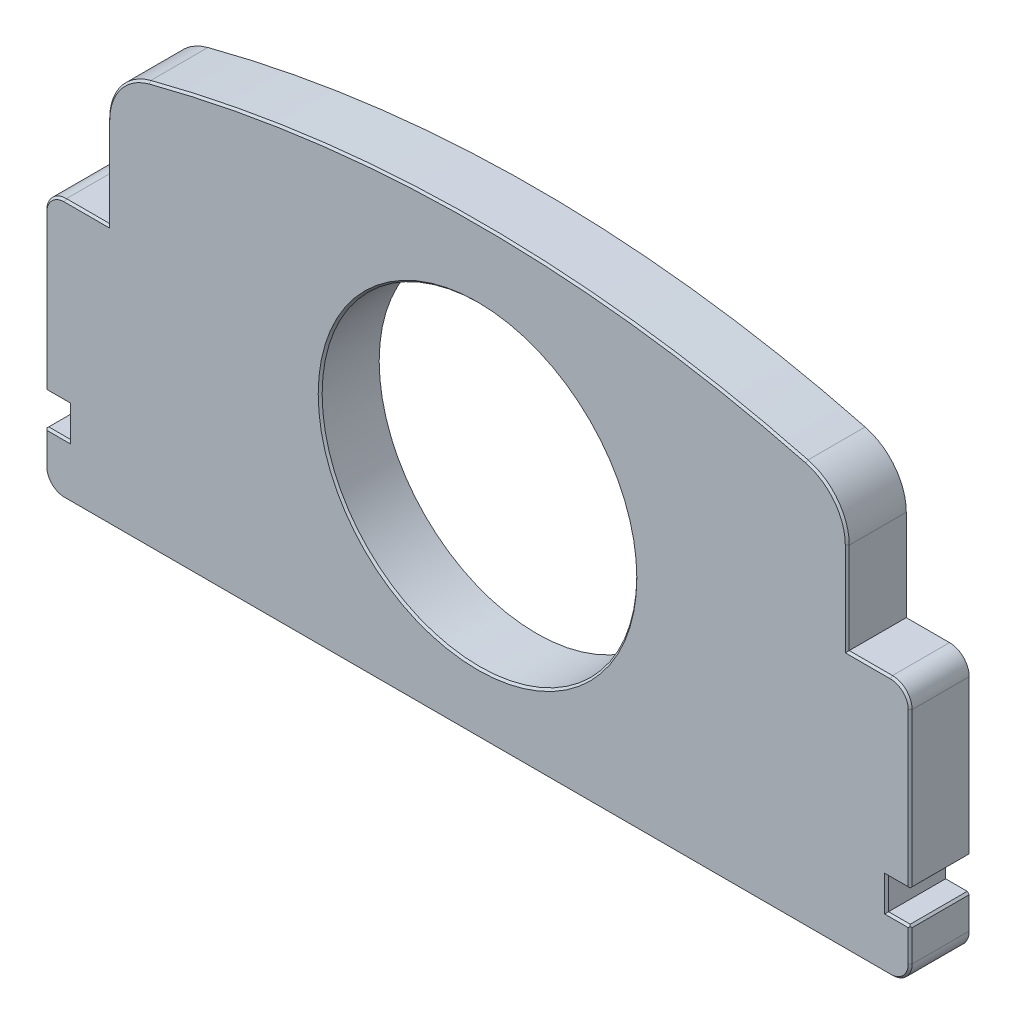
SolidWorks part; units mm, degrees
material "6061 合金"
ref_plane "前视基准面" through (0, 0, 0) normal (0, 0, 1) x (1, 0, 0)
ref_plane "上视基准面" through (0, 0, 0) normal (0, 1, 0) x (1, 0, 0)
ref_plane "右视基准面" through (0, 0, 0) normal (1, 0, 0) x (0, 0, -1)
sketch "草图1" plane through (0, 0, 0) normal (0, 0, 1) x (1, 0, 0)
  line L1 (-110, 121) -> (110, 121)
  line L2 (-110, 121) -> (-110, 0)
  line L3 (-110, 0) -> (110, 0)
  line L4 (110, 121) -> (110, 0)
  dimension "D1" = 220
  dimension "D2" = 121
extrude "凸台-拉伸1" add sketch "草图1" along normal mid plane 15
sketch "草图4" plane through (0, 0, 7.5) normal (0, 0, 1) x (1, 0, 0)
  line L0 (-94, 66) -> (-110, 66)
  line L1 (-110, 121) -> (-110, 0) construction
  line L2 (-110, 122.2) -> (110, 122.2)
  line L3 (110, 122.2) -> (110, 66)
  line L4 (110, 0) -> (110, 121) construction
  line L5 (-94, 66) -> (-94, 89.2057)
  line L6 (94, 66) -> (94, 89.2057)
  line L10 (0, 0) -> (0, 121) construction
  line L12 (110, 66) -> (94, 66)
  line L13 (-110, 66) -> (-110, 122.2)
  line L14 (-110, 0) -> (110, 0) construction
  line L15 (110, 121) -> (-110, 121) construction
  arc A1 (-83.5443, 102.7497) -> (-94, 89.2057) centre (-80, 89.2057) ccw
  arc A2 (83.5443, 102.7497) -> (94, 89.2057) centre (80, 89.2057) cw
  arc A3 (83.5443, 102.7497) -> (-83.5443, 102.7497) centre (0, -216.5) ccw
  dimension "D3" = 14
  dimension "D6" = 330
  dimension "D1" = 66
  dimension "D2" = 188
  dimension "D4" = 56.2
  dimension "D11" = 216.5
sketch "草图5" plane through (0, 0, 7.5) normal (0, 0, 1) x (1, 0, 0)
  line L0 (-110, 121) -> (-110, 0) construction
  line L1 (-110, 21.5) -> (-104, 21.5)
  line L2 (-110, 21.5) -> (-110, 13.5)
  line L3 (-110, 13.5) -> (-104, 13.5)
  line L4 (-104, 21.5) -> (-104, 13.5)
  line L5 (110, 0) -> (110, 121) construction
  line L6 (110, 21.5) -> (104, 21.5)
  line L7 (110, 21.5) -> (110, 13.5)
  line L8 (110, 13.5) -> (104, 13.5)
  line L9 (104, 21.5) -> (104, 13.5)
  line L10 (0, 0) -> (0, 121) construction
  line L11 (110, 121) -> (-110, 121) construction
  line L12 (104, 17.5) -> (-104, 17.5) construction
  line L13 (-110, 0) -> (110, 0) construction
  dimension "D1" = 17.5
  dimension "D2" = 8
  dimension "D3" = 208
extrude "切除-拉伸2" cut sketch "草图5" against normal through all
sketch "草图9" plane through (0, 0, -7.5) normal (0, 0, -1) x (-1, 0, 0)
  line L0 (0, 0) -> (0, 66.5) construction
  line L1 (110, 0) -> (-110, 0) construction
  circle A0 centre (0, 66.5) radius 22.5
  dimension "D2" = 45
  dimension "D1" = 66.5
extrude "切除-拉伸5" cut sketch "草图9" against normal blind 10
extrude "切除-拉伸12" cut sketch "草图4" against normal through all
fillet "圆角1" radius 5 4 edges at (110, 0, 0) (-110, 0, 0) (110, 66, 0) (-110, 66, 0)
chamfer "倒角1" distance 0.5 angle 45 22 edges at (0, 113.5, 7.5) (-91.082, 97.7608, 7.5) (-94, 77.6029, 7.5) (-99.5, 66, 7.5) (-108.5355, 64.5355, 7.5) (-110, 41.25, 7.5) (-107, 21.5, 7.5) (-104, 17.5, 7.5) (-107, 13.5, 7.5) (-110, 9.25, 7.5) (-108.5355, 1.4645, 7.5) (0, 0, 7.5) (108.5355, 1.4645, 7.5) (110, 9.25, 7.5) (107, 13.5, 7.5) (104, 17.5, 7.5) (107, 21.5, 7.5) (110, 41.25, 7.5) (108.5355, 64.5355, 7.5) (99.5, 66, 7.5) (94, 77.6029, 7.5) (91.082, 97.7608, 7.5)
sketch "草图19" plane through (0, 0, 7.5) normal (0, 0, 1) x (1, 0, 0)
  line L0 (0, 55.5) -> (0, 0) construction
  circle A0 centre (0, 55.5) radius 40
  dimension "D1" = 80
  dimension "D2" = 55.5
extrude "切除-拉伸13" cut sketch "草图19" against normal through all
hole_wizard "大小mm 暗销孔1" positions "草图18" profile "草图17" hole size "Ø5.0" standard "GB"
sketch "草图18" plane through (0, 0, -7.5) normal (0, 0, -1) x (-1, 0, 0)
  line L0 (-40, 55.5) -> (40, 55.5) construction
  line L6 (0, 95.5) -> (0, 55.5) construction
  circle A2 centre (0, 55.5) radius 40 construction
  point P0 (-40, 55.5)
  point P2 (40, 55.5)
  dimension "D1" = 80
sketch "草图17" plane through (40, 55.5, -7.5) normal (1, 0, 0) x (0, 1, 0)
  line L0 (0, 0) -> (0, 7.5022)
  line L1 (0, 7.5022) -> (2.5, 6)
  line L2 (2.5, 6) -> (2.5, 0)
  line L5 (2.5, 0) -> (0, 0)
  line L10 (0, 7.5022) -> (-2.5, 6) construction
  line L11 (0, -6.35) -> (0, 107.95) construction
  dimension "孔直径" = 5
  dimension "孔深度" = 6
  dimension "导头角度" = 118
chamfer "倒角2" distance 0.5 angle 45 1 edges at (40, 55.5, 7.5)
chamfer "倒角4" distance 0.5 angle 45 4 edges at (110, 13.5, -0.25) (110, 21.5, -0.25) (-110, 13.5, -0.25) (-110, 21.5, -0.25)
